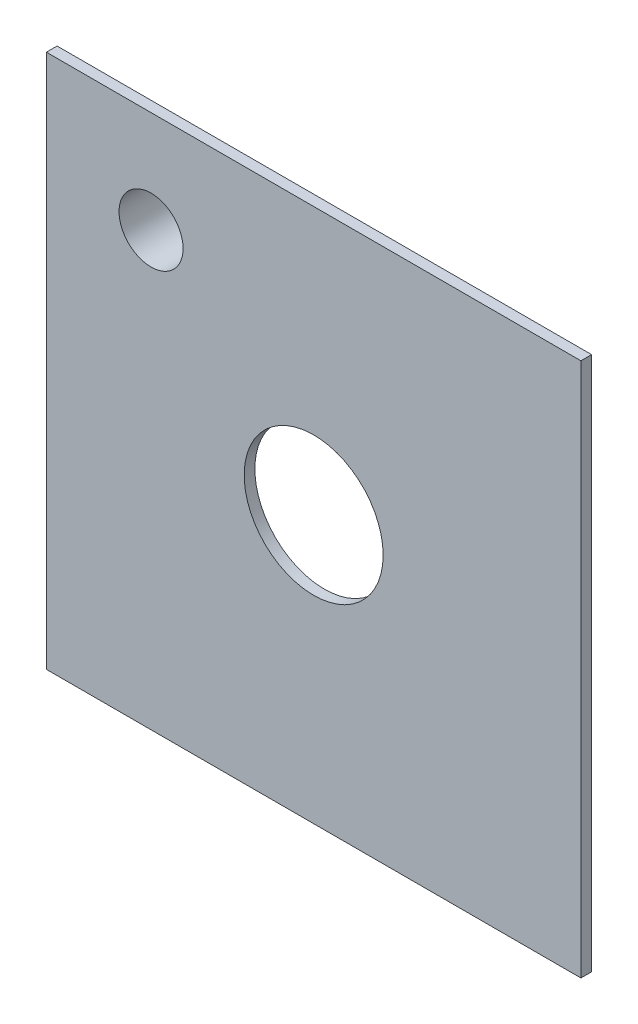
SolidWorks part; units mm, degrees
ref_plane "Front Plane" through (0, 0, 0) normal (0, 0, 1) x (1, 0, 0)
ref_plane "Top Plane" through (0, 0, 0) normal (0, 1, 0) x (1, 0, 0)
ref_plane "Right Plane" through (0, 0, 0) normal (1, 0, 0) x (0, 0, -1)
other "Configuration Table"
sketch "Sketch1" plane through (0, 0, 0) normal (0, 0, 1) x (1, 0, 0)
  line L1 (0, 0) -> (500, 0)
  line L2 (0, 0) -> (0, 500)
  line L3 (0, 500) -> (500, 500)
  line L4 (500, 0) -> (500, 500)
  circle A4 centre (250, 250) radius 65
  circle A5 centre (97.9135, 404.8517) radius 30
  point P7 (0, 0)
  point P10 (500, 0)
  point P15 (0, 500)
  dimension "D4" = 130
  dimension "D5" = 250
  dimension "D6" = 250
  dimension "D7" = 60
  dimension "D1" = 500
  dimension "D2" = 500
extrude "Boss-Extrude1" add sketch "Sketch1" along normal blind 10
sketch "Sketch2" plane through (0, 0, 10) normal (0, 0, 1) x (1, 0, 0)
  circle A0 centre (97.9135, 404.8517) radius 29.9571
  circle A1 centre (97.9135, 404.8517) radius 35
  dimension "D1" = 70
extrude "Boss-Extrude2" add sketch "Sketch2" against normal blind 50
